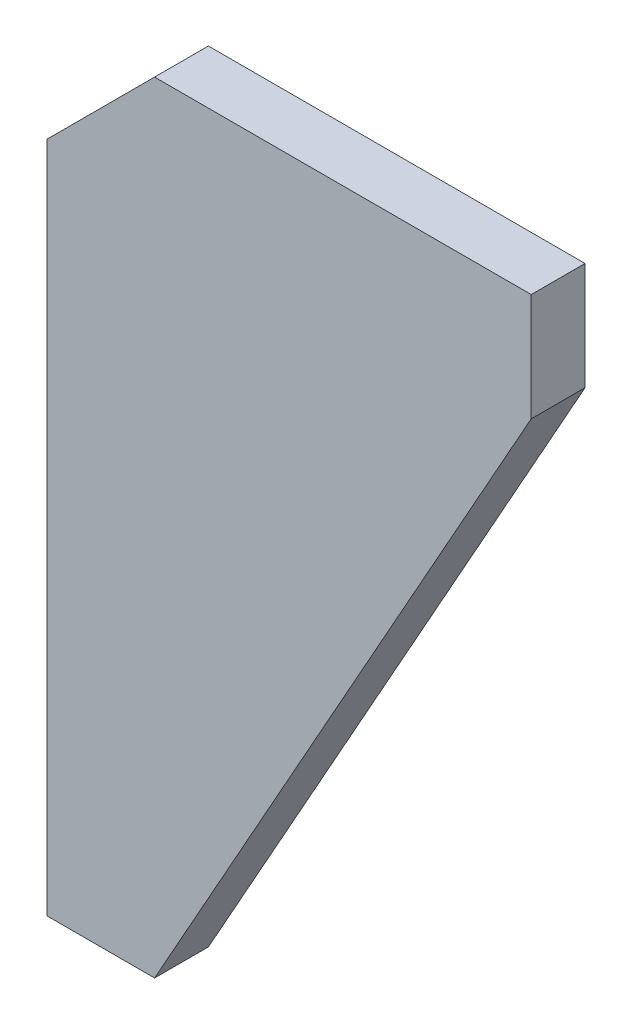
SolidWorks part; units mm, degrees
material "Q235"
ref_plane "Front Plane" through (0, 0, 0) normal (0, 0, 1) x (1, 0, 0)
ref_plane "Top Plane" through (0, 0, 0) normal (0, 1, 0) x (1, 0, 0)
ref_plane "Right Plane" through (0, 0, 0) normal (1, 0, 0) x (0, 0, -1)
sketch "Sketch1" plane through (0, 0, 0) normal (0, 0, 1) x (1, 0, 0)
  line L0 (0, 0) -> (20, 0)
  line L1 (20, 0) -> (90, 125)
  line L2 (90, 125) -> (90, 145)
  line L3 (90, 145) -> (20, 145)
  line L4 (20, 145) -> (0, 125)
  line L5 (0, 125) -> (0, 0)
  dimension "D1" = 145
  dimension "D2" = 90
  dimension "D3" = 20
  dimension "D4" = 20
  dimension "D5" = 20
  dimension "D6" = 20
extrude "Boss-Extrude1" add sketch "Sketch1" along normal blind 10
sketch "Sketch3" plane through (0, 0, 0) normal (-1, 0, 0) x (0, 0, 1)
  line L0 (5, 0) -> (5, 125) construction
  line L1 (10, 0) -> (0, 0) construction
  line L2 (10, 125) -> (0, 125) construction
